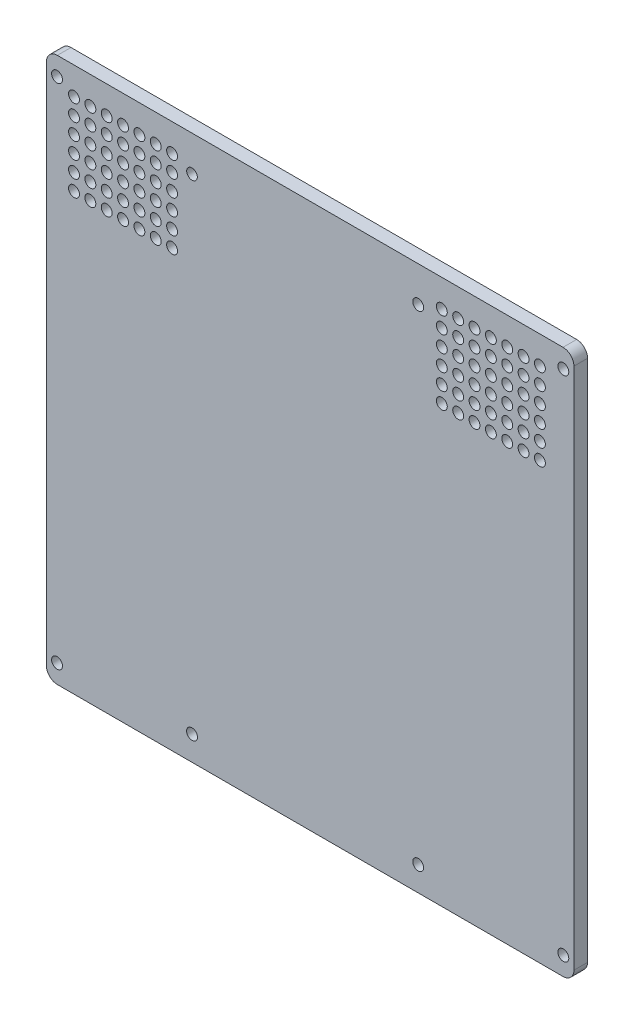
SolidWorks part; units mm, degrees
ref_plane "Front Plane" through (0, 0, 0) normal (0, 0, 1) x (1, 0, 0)
ref_plane "Top Plane" through (0, 0, 0) normal (0, 1, 0) x (1, 0, 0)
ref_plane "Right Plane" through (0, 0, 0) normal (1, 0, 0) x (0, 0, -1)
sketch "Sketch1" plane through (0, 0, 0) normal (0, 0, 1) x (1, 0, 0)
  line L5 (-38.6, 12.1212) -> (155, 12.1212)
  line L6 (-38.6, 12.1212) -> (-38.6, -187.8788)
  line L7 (-38.6, -187.8788) -> (155, -187.8788)
  line L8 (155, 12.1212) -> (155, -187.8788)
  dimension "D1" = 193.6
  dimension "D2" = 200
extrude "Boss-Extrude1" add sketch "Sketch1" along normal blind 5
sketch "Sketch2" plane through (0, 0, 5) normal (0, 0, 1) x (1, 0, 0)
sketch "Sketch3" plane through (0, 0, 5) normal (0, 0, 1) x (1, 0, 0)
  circle A0 centre (97.8413, -178.911) radius 2
  circle A2 centre (97.8413, -0.893) radius 2
  circle A4 centre (14.827, -178.911) radius 2
  circle A5 centre (14.827, -0.893) radius 1.9524
  dimension "D1" = 4
  dimension "D2" = 4
  dimension "D3" = 4
extrude "Cut-Extrude2" cut sketch "Sketch3" against normal blind 12
sketch "Sketch4" plane through (0, 0, 5) normal (0, 0, 1) x (1, 0, 0)
  line L0 (58.2, -187.8788) -> (58.2, 12.1212) construction
  line L1 (-38.6, -187.8788) -> (155, -187.8788) construction
  line L2 (155, 12.1212) -> (-38.6, 12.1212) construction
  circle A0 centre (151.1094, -181.0431) radius 2
  circle A1 centre (151.1094, 5.2855) radius 2
  circle A2 centre (-34.7094, 5.2855) radius 2
  circle A3 centre (-34.7094, -181.0431) radius 2
  dimension "D1" = 4
extrude "Cut-Extrude3" cut sketch "Sketch4" against normal blind 10
fillet "Fillet1" radius 4 4 edges at (-38.6, 12.1212, 2.5) (155, 12.1212, 2.5) (-38.6, -187.8788, 2.5) (155, -187.8788, 2.5)
sketch "Sketch5" plane through (0, 0, 5) normal (0, 0, 1) x (1, 0, 0)
  circle A0 centre (142.5154, 1.9818) radius 2
  circle A1 centre (136.5154, 1.9818) radius 2
  circle A2 centre (130.5154, 1.9818) radius 2
  circle A3 centre (124.5154, 1.9818) radius 2
  circle A4 centre (118.5154, 1.9818) radius 2
  circle A5 centre (112.5154, 1.9818) radius 2
  circle A6 centre (106.5154, 1.9818) radius 2
  circle A7 centre (136.5154, -4.0182) radius 2
  circle A8 centre (130.5154, -4.0182) radius 2
  circle A9 centre (124.5154, -4.0182) radius 2
  circle A10 centre (118.5154, -4.0182) radius 2
  circle A11 centre (112.5154, -4.0182) radius 2
  circle A12 centre (106.5154, -4.0182) radius 2
  circle A13 centre (136.5154, -10.0182) radius 2
  circle A14 centre (130.5154, -10.0182) radius 2
  circle A15 centre (124.5154, -10.0182) radius 2
  circle A16 centre (118.5154, -10.0182) radius 2
  circle A17 centre (112.5154, -10.0182) radius 2
  circle A18 centre (106.5154, -10.0182) radius 2
  circle A19 centre (136.5154, -16.0182) radius 2
  circle A20 centre (130.5154, -16.0182) radius 2
  circle A21 centre (124.5154, -16.0182) radius 2
  circle A22 centre (118.5154, -16.0182) radius 2
  circle A23 centre (112.5154, -16.0182) radius 2
  circle A24 centre (106.5154, -16.0182) radius 2
  circle A25 centre (136.5154, -22.0182) radius 2
  circle A26 centre (130.5154, -22.0182) radius 2
  circle A27 centre (124.5154, -22.0182) radius 2
  circle A28 centre (118.5154, -22.0182) radius 2
  circle A29 centre (112.5154, -22.0182) radius 2
  circle A30 centre (106.5154, -22.0182) radius 2
  circle A31 centre (136.5154, -28.0182) radius 2
  circle A32 centre (130.5154, -28.0182) radius 2
  circle A33 centre (124.5154, -28.0182) radius 2
  circle A34 centre (118.5154, -28.0182) radius 2
  circle A35 centre (112.5154, -28.0182) radius 2
  circle A36 centre (106.5154, -28.0182) radius 2
  circle A37 centre (142.5154, -4.0182) radius 2
  circle A38 centre (142.5154, -10.0182) radius 2
  circle A39 centre (142.5154, -16.0182) radius 2
  circle A40 centre (142.5154, -22.0182) radius 2
  circle A41 centre (142.5154, -28.0182) radius 2
  dimension "D1" = 4
  dimension "D3" = 6
  dimension "D4" = 6
  dimension "D2" = 6
extrude "Cut-Extrude4" cut sketch "Sketch5" against normal blind 10
pattern_linear "LPattern1" count 2 spacing 135 along (-1, 0, 0) of "Cut-Extrude4"
